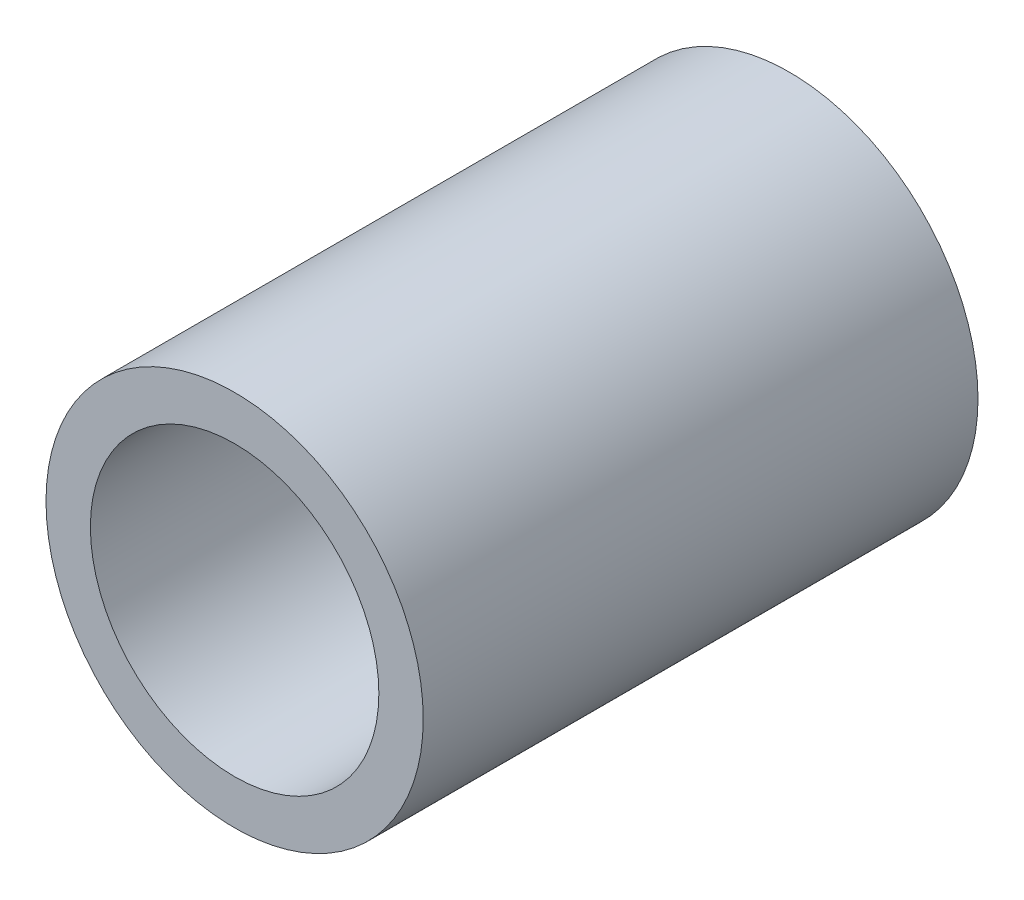
from build123d import *

# Parameters (mm, degrees)
SKETCH1_R           = 17
SKETCH1_R_2         = 13
BOSS_EXTRUDE1_DEPTH = 50


with BuildPart() as part:
    # Sketch1 → Boss-Extrude1 (new body)
    with BuildSketch(Plane.XY):
        Circle(SKETCH1_R)
        Circle(SKETCH1_R_2, mode=Mode.SUBTRACT)
    extrude(amount=BOSS_EXTRUDE1_DEPTH)


solid = part.part
